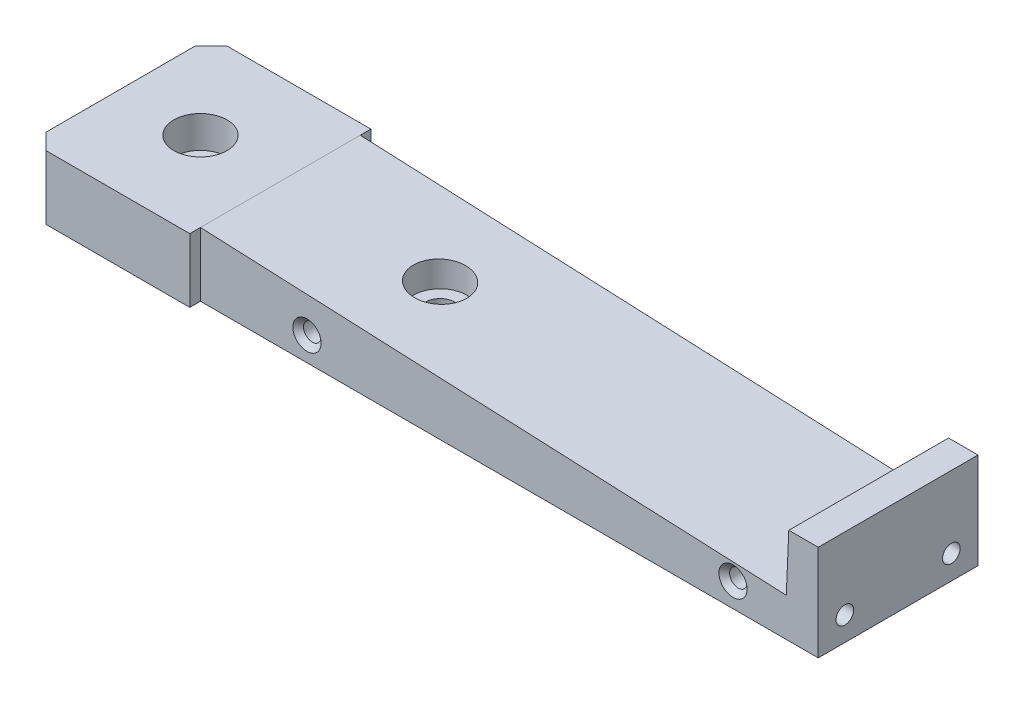
SolidWorks part; units mm, degrees
ref_plane "Front Plane" through (0, 0, 0) normal (0, 0, 1) x (1, 0, 0)
ref_plane "Top Plane" through (0, 0, 0) normal (0, 1, 0) x (1, 0, 0)
ref_plane "Right Plane" through (0, 0, 0) normal (1, 0, 0) x (0, 0, -1)
sketch "Sketch1" plane through (0, 0, 0) normal (0, 1, 0) x (1, 0, 0)
  line L1 (-73, 17) -> (73, 17)
  line L2 (-73, 17) -> (-73, -17)
  line L3 (-73, -17) -> (73, -17)
  line L4 (73, 17) -> (73, -17)
  line L5 (-73, 17) -> (73, -17) construction
  line L6 (-73, -17) -> (73, 17) construction
  point P0 (0, 0)
  dimension "D1" = 34
  dimension "D2" = 146
extrude "Boss-Extrude1" add sketch "Sketch1" along normal mid plane 12
hole_wizard "Hole size per socket head cap screw type1" positions "Sketch3" profile "Sketch2" counterbore size "M5" standard "Gb" end condition through all
sketch "Sketch3" plane through (0, 6, 0) normal (0, 1, 0) x (1, 0, 0)
  line L0 (-73, 17) -> (-73, -17) construction
  point P0 (-58, 0)
  point P2 (-13, 0)
  dimension "D1" = 45
  dimension "D2" = 15
sketch "Sketch2" plane through (-58, 6, 0) normal (1, 0, 0) x (0, 0, 1)
  line L0 (0, 0) -> (0, 12)
  line L1 (0, 12) -> (2.75, 12)
  line L3 (2.75, 12) -> (2.75, 6)
  line L4 (2.75, 6) -> (5, 6)
  line L5 (5, 6) -> (5, 0)
  line L7 (5, 0) -> (0, 0)
  line L11 (0, -6.35) -> (0, 107.95) construction
  dimension "通孔孔直径" = 5.5
  dimension "通孔孔深度" = 12
  dimension "柱形沉头孔直径" = 10
  dimension "柱形沉头孔深度" = 6
hole_wizard "M4 Tapped Hole2" positions "Sketch7" profile "Sketch6" tap size "M4" standard "Gb"
sketch "Sketch7" plane through (73, 0, 0) normal (1, 0, 0) x (0, 0, -1)
  line L0 (0, 0) -> (0, 8.2581) construction
  line L1 (-17, -6) -> (17, -6) construction
  point P0 (-10, -1.5)
  point P2 (10, -1.5)
  dimension "D1" = 20
  dimension "D2" = 4.5
sketch "Sketch6" plane through (73, -1.5, 10) normal (0, 1, 0) x (0, 0, -1)
  line L0 (0, 0) -> (0, 11.0914)
  line L1 (0, 11.0914) -> (1.65, 10.1)
  line L2 (1.65, 10.1) -> (1.65, 0)
  line L5 (1.65, 0) -> (0, 0)
  line L10 (0, 11.0914) -> (-1.65, 10.1) construction
  line L11 (0, -6.35) -> (0, 107.95) construction
  dimension "螺纹孔钻头直径" = 3.3
  dimension "螺纹孔钻头深度" = 10.1
  dimension "导头角度" = 118
cosmetic thread "Cosmetic Thread3" parameters "D1"=8, "D2"=4
cosmetic thread "Cosmetic Thread4" parameters "D1"=8, "D2"=4
chamfer "Chamfer1" distance 3 angle 45 2 edges at (-73, 0, -17) (-73, 0, 17)
sketch "Sketch8" plane through (0, 6, 0) normal (0, 1, 0) x (1, 0, 0)
  line L0 (-73, 14) -> (-73, -14) construction
  line L1 (73, -17) -> (-43, -17)
  line L2 (73, -17) -> (73, -15)
  line L3 (73, -15) -> (-43, -15)
  line L4 (-43, -17) -> (-43, -15)
  line L5 (73, 17) -> (-43, 17)
  line L6 (73, 17) -> (73, 15)
  line L7 (73, 15) -> (-43, 15)
  line L8 (-43, 17) -> (-43, 15)
  dimension "D1" = 30
  dimension "D2" = 2
  dimension "D3" = 2
extrude "Cut-Extrude1" cut sketch "Sketch8" against normal through all
hole_wizard "M4 Tapped Hole3" positions "Sketch10" profile "Sketch9" tap size "M4" standard "Gb"
sketch "Sketch10" plane through (0, 0, 15) normal (0, 0, 1) x (1, 0, 0)
  line L1 (-70, -6) -> (-43, -6) construction
  line L2 (-73, -6) -> (-73, 6) construction
  point P0 (-23, -1.5)
  point P3 (57, -1.5)
  dimension "D1" = 80
  dimension "D2" = 50
  dimension "D3" = 4.5
sketch "Sketch9" plane through (-23, -1.5, 15) normal (1, 0, 0) x (0, -1, 0)
  line L0 (0, 0) -> (0, 11.0914)
  line L1 (0, 11.0914) -> (1.65, 10.1)
  line L2 (1.65, 10.1) -> (1.65, 0)
  line L5 (1.65, 0) -> (0, 0)
  line L10 (0, 11.0914) -> (-1.65, 10.1) construction
  line L11 (0, -6.35) -> (0, 107.95) construction
  dimension "螺纹孔钻头直径" = 3.3
  dimension "螺纹孔钻头深度" = 10.1
  dimension "导头角度" = 118
cosmetic thread "Cosmetic Thread5" parameters "D1"=8, "D2"=4
cosmetic thread "Cosmetic Thread6" parameters "D1"=8, "D2"=4
mirror "Mirror1" about plane through (0, 0, 0) normal (0, 0, 1) of "M4 Tapped Hole3"
sketch "Sketch11" plane through (0, 6, 0) normal (0, 1, 0) x (1, 0, 0)
  line L0 (-43, 15) -> (73, 15) construction
  line L1 (73, -15) -> (67, -15)
  line L2 (73, -15) -> (73, 15)
  line L3 (73, 15) -> (67, 15)
  line L4 (67, -15) -> (67, 15)
  dimension "D1" = 6
extrude "Boss-Extrude2" add sketch "Sketch11" along normal blind 6
sketch "Sketch12" plane through (0, 0, 17) normal (0, 0, 1) x (1, 0, 0)
  line L0 (67, 6) -> (-43, 6) construction
  line L1 (67, 6) -> (-43, 6)
  line L2 (-43, 6) -> (67, 1.1973)
  line L4 (67, 6) -> (67, 1.1973)
  dimension "D1" = 2.5
extrude "Cut-Extrude2" cut sketch "Sketch12" against normal through all
sketch "Sketch13" plane through (0, 0, 17) normal (0, 0, 1) x (1, 0, 0)
  line L0 (67, 12) -> (67, 1.1973) construction
  line L1 (67, 12) -> (67, 1.1973)
  line L2 (67, 1.1973) -> (67.4717, 12)
  line L4 (67, 12) -> (73, 12) construction
  line L5 (67, 12) -> (67.4717, 12)
  dimension "D1" = 2.5
extrude "Cut-Extrude3" cut sketch "Sketch13" against normal through all
chamfer "Chamfer2" distance 1 angle 45 4 edges at (-24.65, -1.5, -15) (55.35, -1.5, -15) (58.65, -1.5, 15) (-21.35, -1.5, 15)
